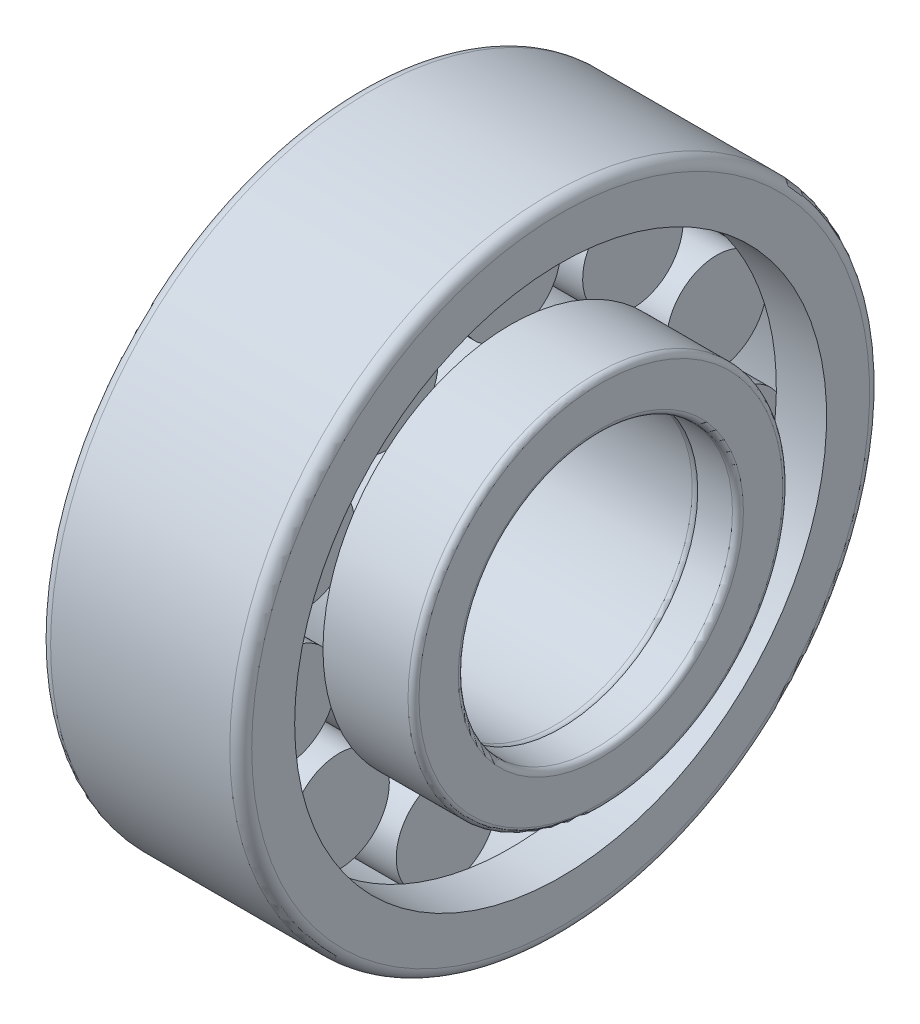
SolidWorks part; units mm, degrees
revolve "基体-旋转" add sketch "草图2" angle 360 about L0
sketch "草图2" plane through (0, 0, 0) normal (0, 0, 1) x (1, 0, 0)
  line L0 (-10.0801, 0) -> (21.9267, 0) construction
  line L1 (2.75, 9.65) -> (8.25, 9.65)
  line L2 (0, 10.25) -> (2.75, 10.25)
  line L3 (0, 10.25) -> (0, 7.8)
  line L4 (0.3, 7.5) -> (10.7, 7.5)
  line L5 (11, 8.9131) -> (11, 7.8)
  line L6 (2.75, 9.65) -> (2.75, 10.25)
  line L7 (11, 8.9131) -> (8.25, 9.65)
  arc A0 (10.7, 7.5) -> (11, 7.8) centre (10.7, 7.8) ccw
  arc A1 (0, 7.8) -> (0.3, 7.5) centre (0.3, 7.8) ccw
  point P13 (11, 7.5)
  point P16 (0, 7.5)
revolve "凸台-旋转1" add sketch "草图3" angle 360 about L2
sketch "草图3" plane through (0, 0, 0) normal (0, 0, 1) x (1, 0, 0)
  line L1 (8.25, 9.65) -> (8.25, -9.65) construction
  line L2 (-1.6039, 12.4) -> (13.5036, 12.4) construction
  line L4 (2.75, 12.4) -> (8.25, 12.4)
  line L5 (2.75, 12.4) -> (2.75, 9.6499)
  line L6 (2.75, 9.6499) -> (8.25, 9.6499)
  line L7 (8.25, 12.4) -> (8.25, 9.6499)
  line L8 (2.75, -10.25) -> (2.75, 10.25) construction
  dimension "D1" = 12.4
  dimension "D2" = 2.7501
revolve "凸台-旋转2" add sketch "草图4" angle 360 about L0
sketch "草图4" plane through (0, 0, 0) normal (0, 0, 1) x (1, 0, 0)
  line L0 (0, 0) -> (17.8006, 0) construction
  line L1 (-10.0801, 0) -> (21.9267, 0) construction
  line L2 (8.25, 14.55) -> (11, 14.55)
  line L3 (0.6, 17.5) -> (10.4, 17.5)
  line L4 (0, 16.9) -> (0, 14.55)
  line L5 (0, 14.55) -> (2.75, 14.55)
  line L6 (11, 16.9) -> (11, 14.55)
  line L7 (2.75, 15.15) -> (8.25, 15.15)
  line L8 (2.75, 15.15) -> (2.75, 14.55)
  line L10 (8.25, 15.15) -> (8.25, 14.55)
  arc A0 (10.4, 17.5) -> (11, 16.9) centre (10.4, 16.9) cw
  arc A1 (0.6, 17.5) -> (0, 16.9) centre (0.6, 16.9) ccw
  point P15 (11, 17.5)
  point P18 (0, 17.5)
material "GCr4"
ref_plane "基准面1" through (0, 0, 0) normal (0, 0, 1) x (1, 0, 0)
ref_plane "基准面2" through (0, 0, 0) normal (0, 1, 0) x (1, 0, 0)
ref_plane "基准面3" through (0, 0, 0) normal (1, 0, 0) x (0, 0, -1)
sketch "尺寸草图" plane through (0, 0, 0) normal (0, 0, 1) x (1, 0, 0)
  line L0 (0, 0) -> (0.3, 0)
  line L1 (0.3, 0) -> (0.9, 0)
  line L2 (0.9, 0) -> (11.9, 0)
  line L3 (11.9, 0) -> (26.9, 0)
  line L4 (26.9, 0) -> (46.2, 0)
  line L5 (46.2, 0) -> (81.2, 0)
  line L6 (111.5, 0) -> (113.7, 0)
  line L7 (81.2, 0) -> (111.5, 0)
sketch "草图5" plane through (0, 0, 0) normal (0, 0, 1) x (1, 0, 0)
  line L0 (0, 0) -> (19.6659, 0) construction
  line L1 (-10.0801, 0) -> (21.9267, 0) construction
  line L2 (11, 8.9131) -> (11, 7.5)
  line L3 (11, -8.9131) -> (11, 8.9131) construction
  line L4 (11, -7.8) -> (11, 7.8) construction
  line L5 (11, 8.9131) -> (8.25, 9.65)
  line L6 (11, -14.55) -> (11, 14.55) construction
  line L7 (8.25, 9.65) -> (8.25, 10.25)
  line L8 (8.25, 10.25) -> (12.9, 10.25)
  line L9 (13.2, 9.95) -> (13.2, 7.8)
  line L10 (12.9, 7.5) -> (11, 7.5)
  arc A0 (12.9, 10.25) -> (13.2, 9.95) centre (12.9, 9.95) cw
  arc A1 (12.9, 7.5) -> (13.2, 7.8) centre (12.9, 7.8) ccw
revolve "凸台-旋转3" add sketch "草图5" angle 360 about L0
pattern_circular "阵列(圆周)1" count 11 over 360 about axis through (0, 0, 0) along (1, 0, 0) of "凸台-旋转1"
equation "\"DD@草图2\" = \"内径@尺寸草图\""
equation "\"FW@草图2\" = \"参考FW@尺寸草图\""
equation "\"D1@草图2\" = \"倒角小@尺寸草图\""
equation "\"EW@草图4\" = \"参考EW@尺寸草图\""
equation "\"B@草图4\" = \"宽度@尺寸草图\""
equation "\"D@草图4\" = \"外径@尺寸草图\""
equation "\"D2@草图4\" = \"倒角大@尺寸草图\""
equation "\"架宽度@尺寸草图\" = 0.20*\"宽度@尺寸草图\""
equation "\"D5@草图5\" = \"架宽度@尺寸草图\""
equation "\"D4@草图2\" = \"FW@草图2\" + 4 *\"D1@草图2\""
equation "\"D2@草图2\" = \"B@草图4\""
equation "\"滚珠位置@草图2\" = \"D2@草图2\"/4"
equation "\"D3@草图4\" = \"D2@草图4\""
equation "\"D1@草图3\" =  ( \"EW@草图4\" - \"FW@草图2\" )  / 4 + \"FW@草图2\" / 2"
equation "\"D2@草图3\" =  0.25*( \"EW@草图4\" - \"FW@草图2\" ) +0.0001"
equation "\"D1@阵列(圆周)1\" =0.75* \"D1@草图3\" * 3.14 / \"D2@草图3\""
equation "\"D1@草图5\" = \"D1@草图2\""
equation "\"D4@草图5\" = \"D4@草图2\""
equation "\"D2@草图5\" = \"DD@草图2\""
